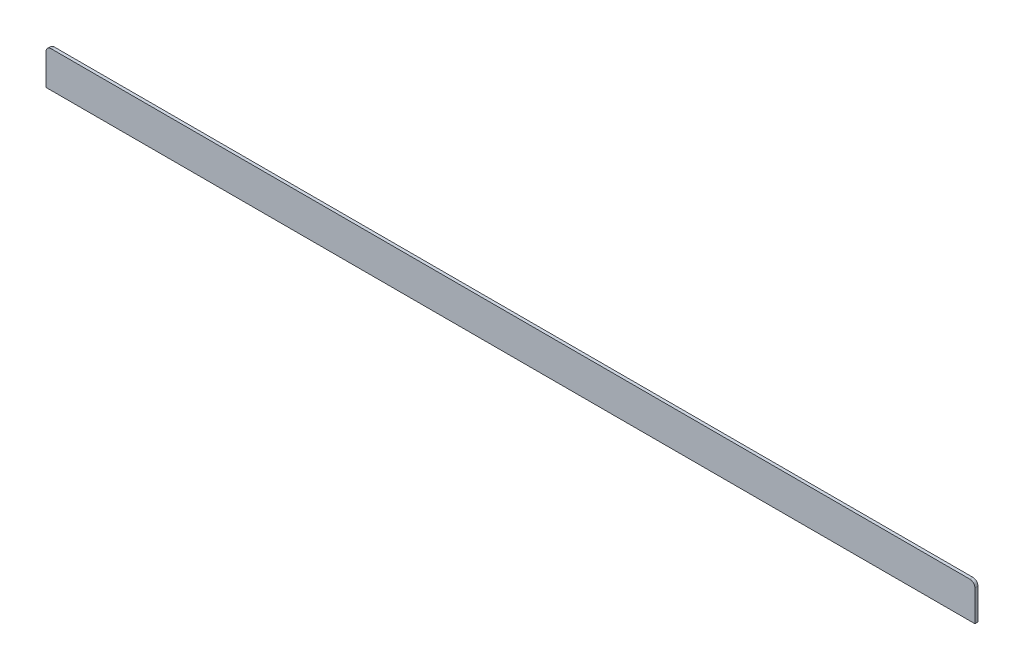
from build123d import *

# Parameters (mm, degrees)
SKETCH_1_W      = 900
SKETCH_1_H      = 35
EXTRUDE_1_DEPTH = 3
FILLET_1_R      = 5


with BuildPart() as part:
    # 草图1 → 凸台-拉伸1 (new body)
    with BuildSketch(Plane.XY):
        Rectangle(SKETCH_1_W, SKETCH_1_H)
    extrude(amount=EXTRUDE_1_DEPTH)

    # 圆角1
    fillet_1_edges = [part.edges().sort_by_distance(p)[0] for p in [
        (-450, 17.5, 1.5),
        (450, 17.5, 1.5),
    ]]
    fillet(fillet_1_edges, radius=FILLET_1_R)


solid = part.part
